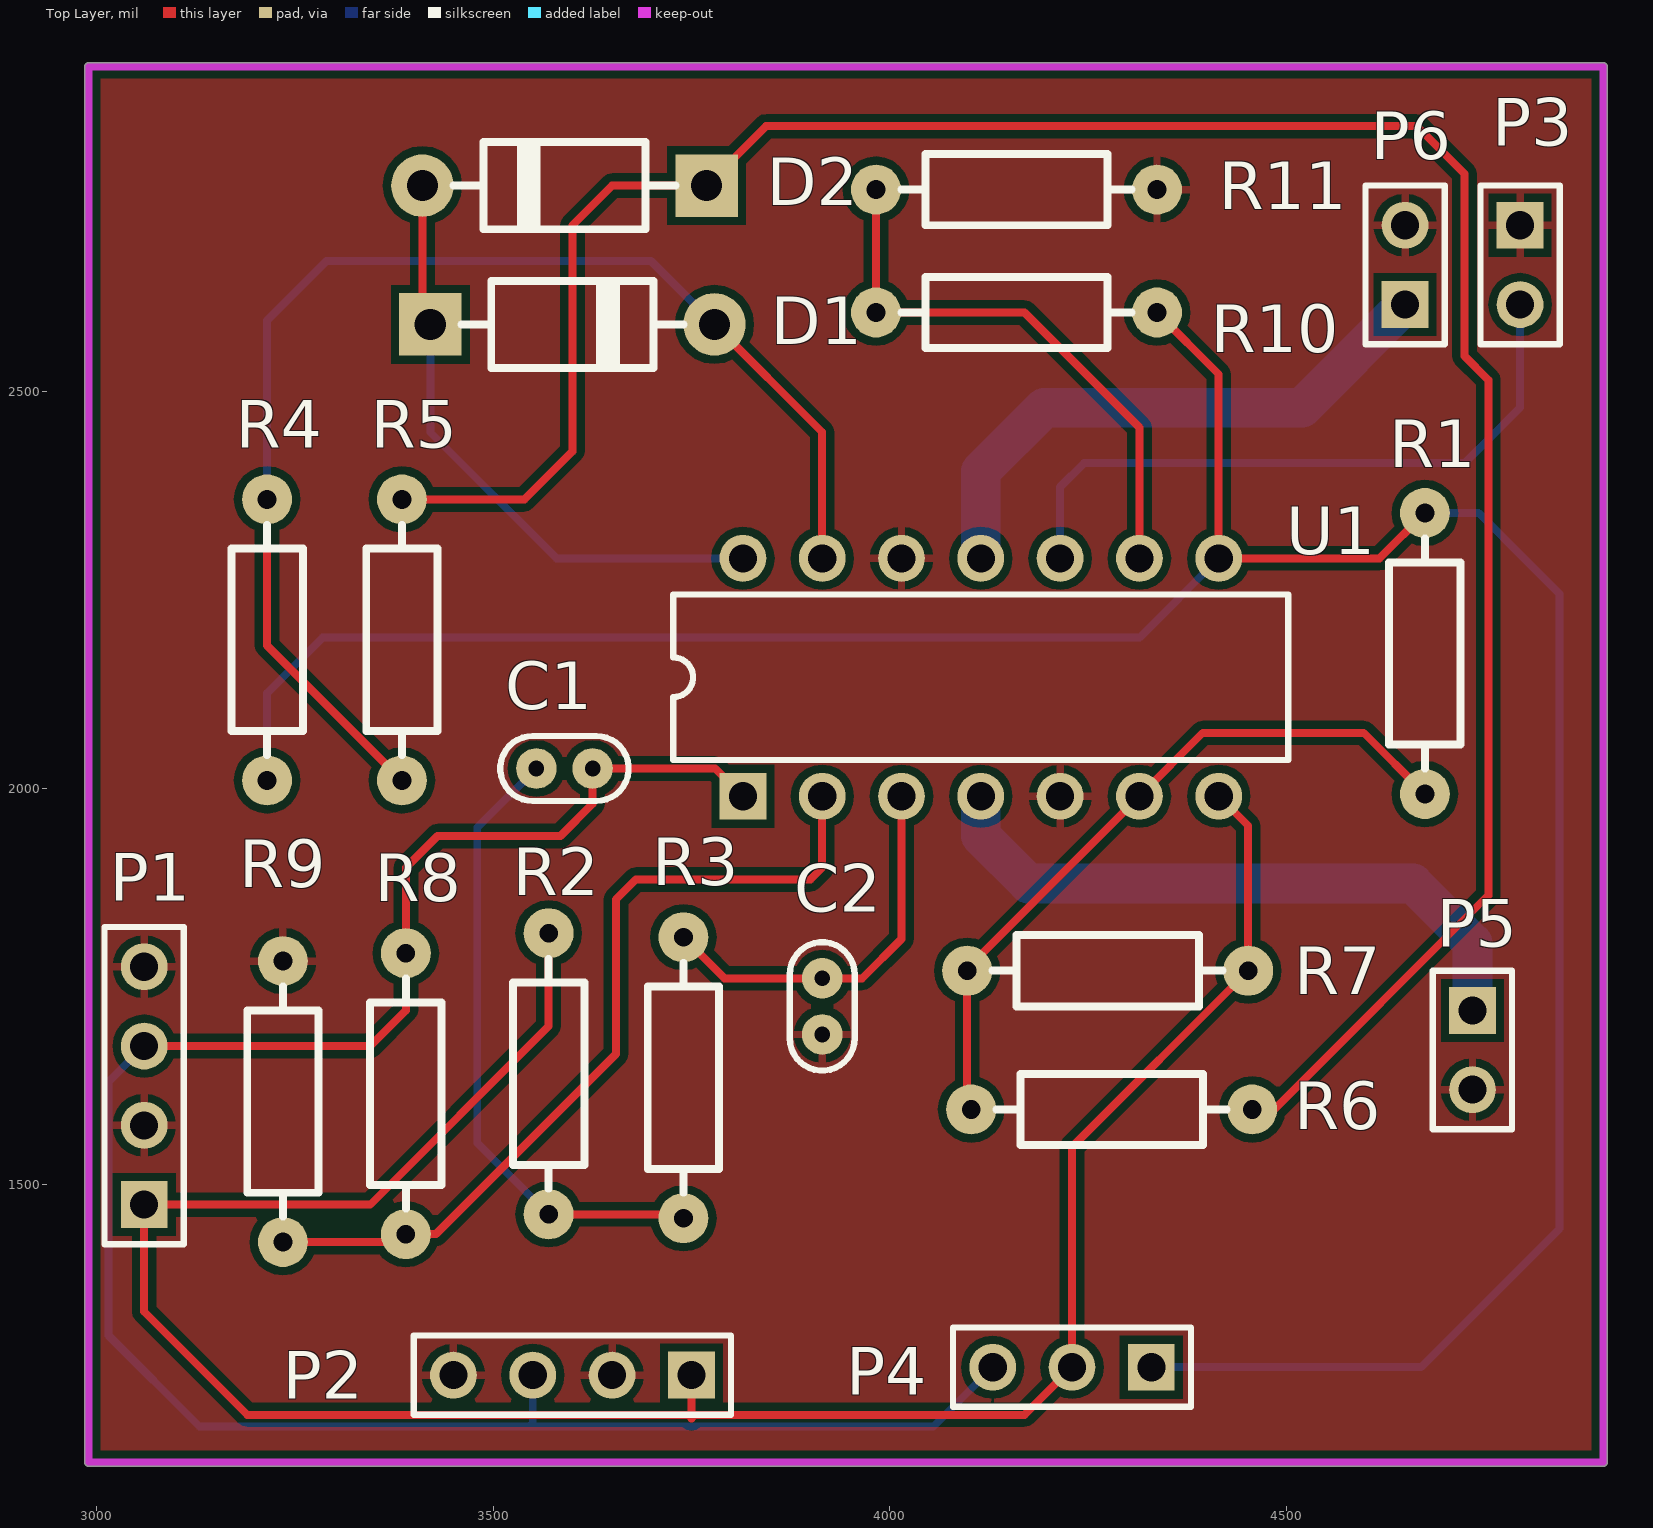
[diagram p0: Top Layer view]
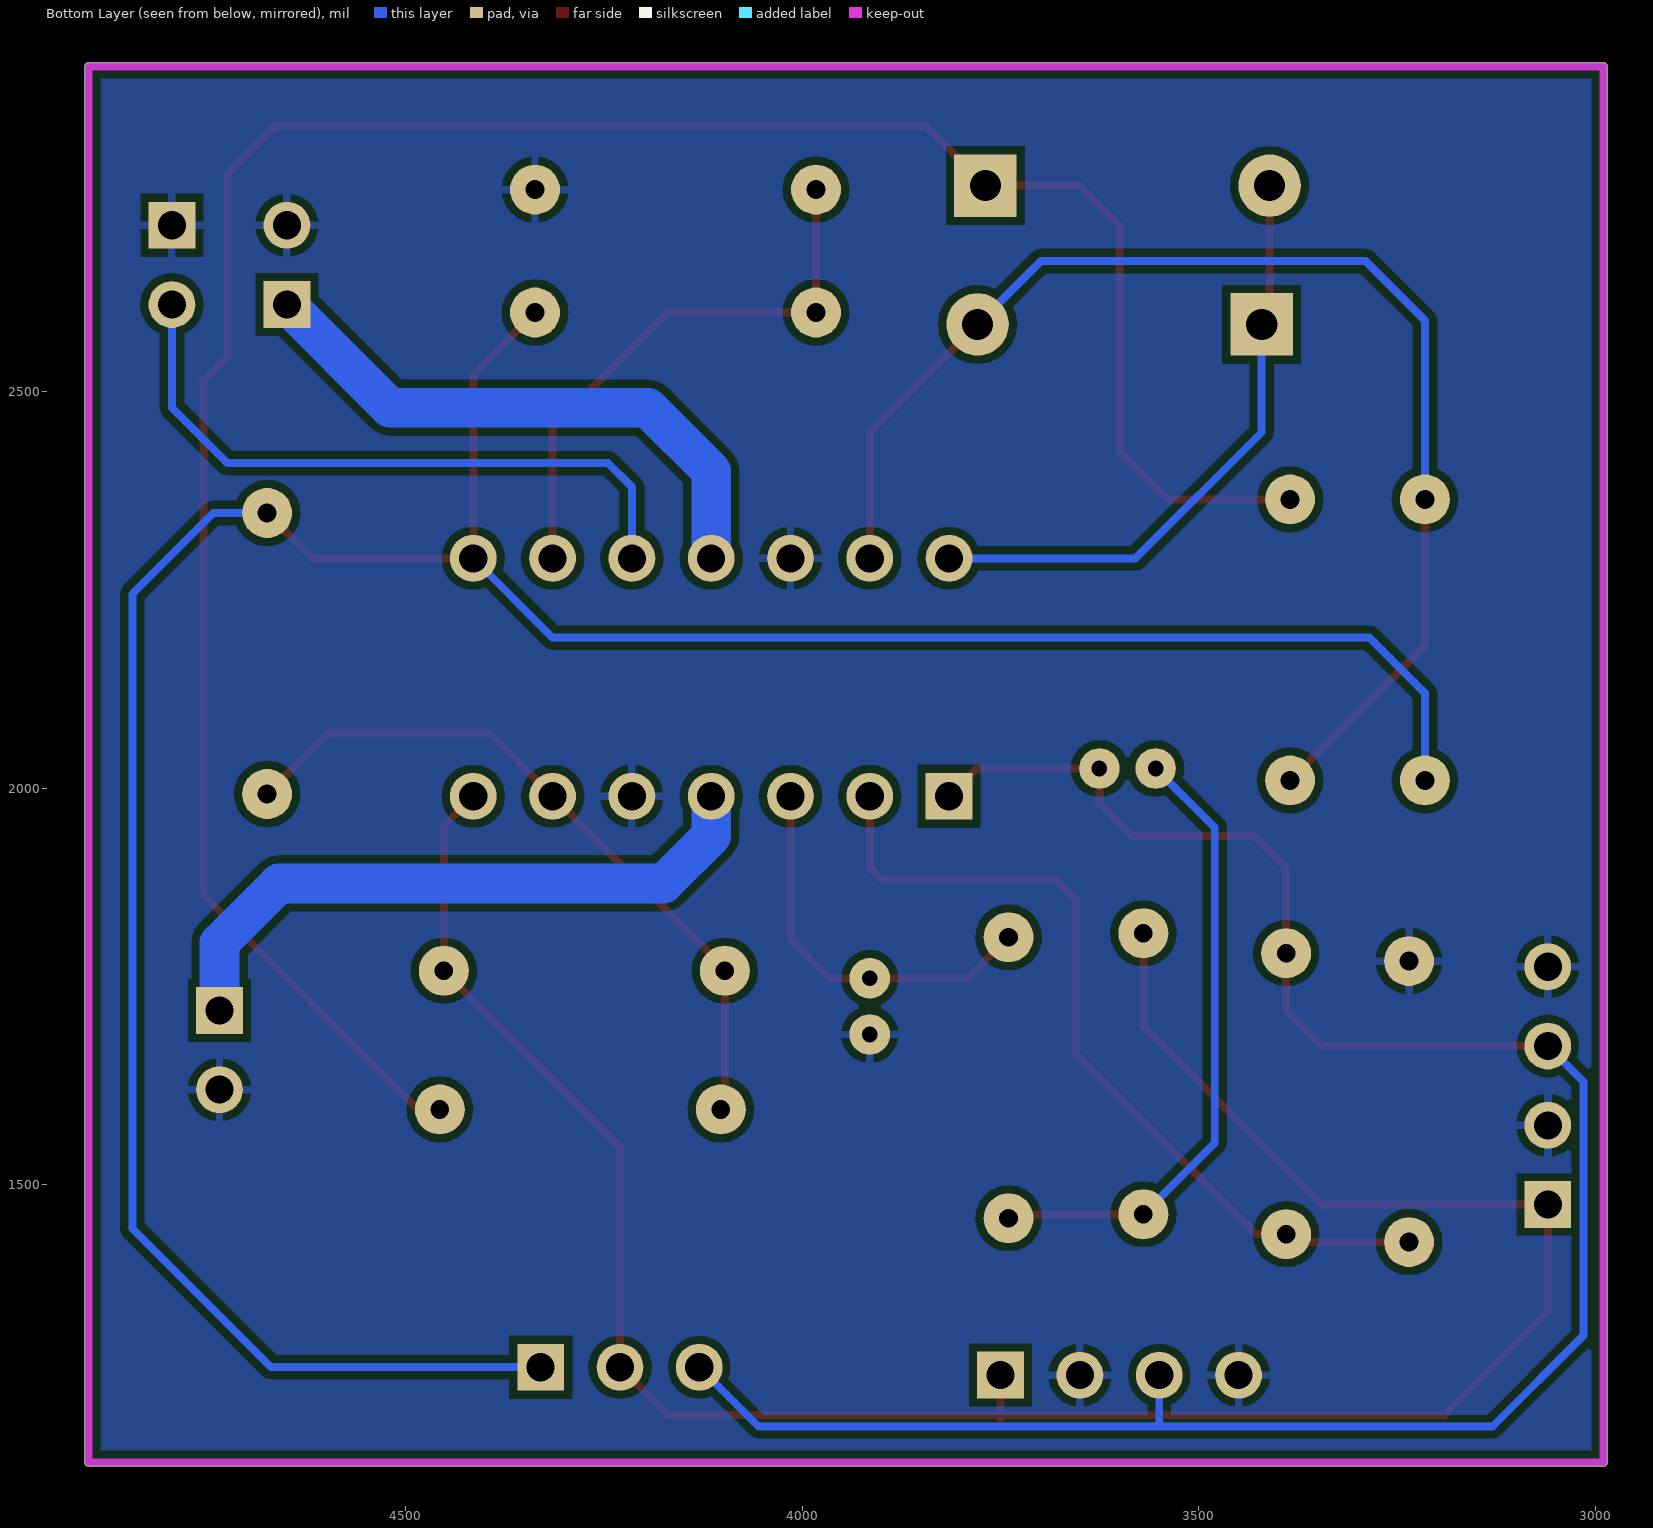
[diagram p1: Bottom Layer view, seen from below]
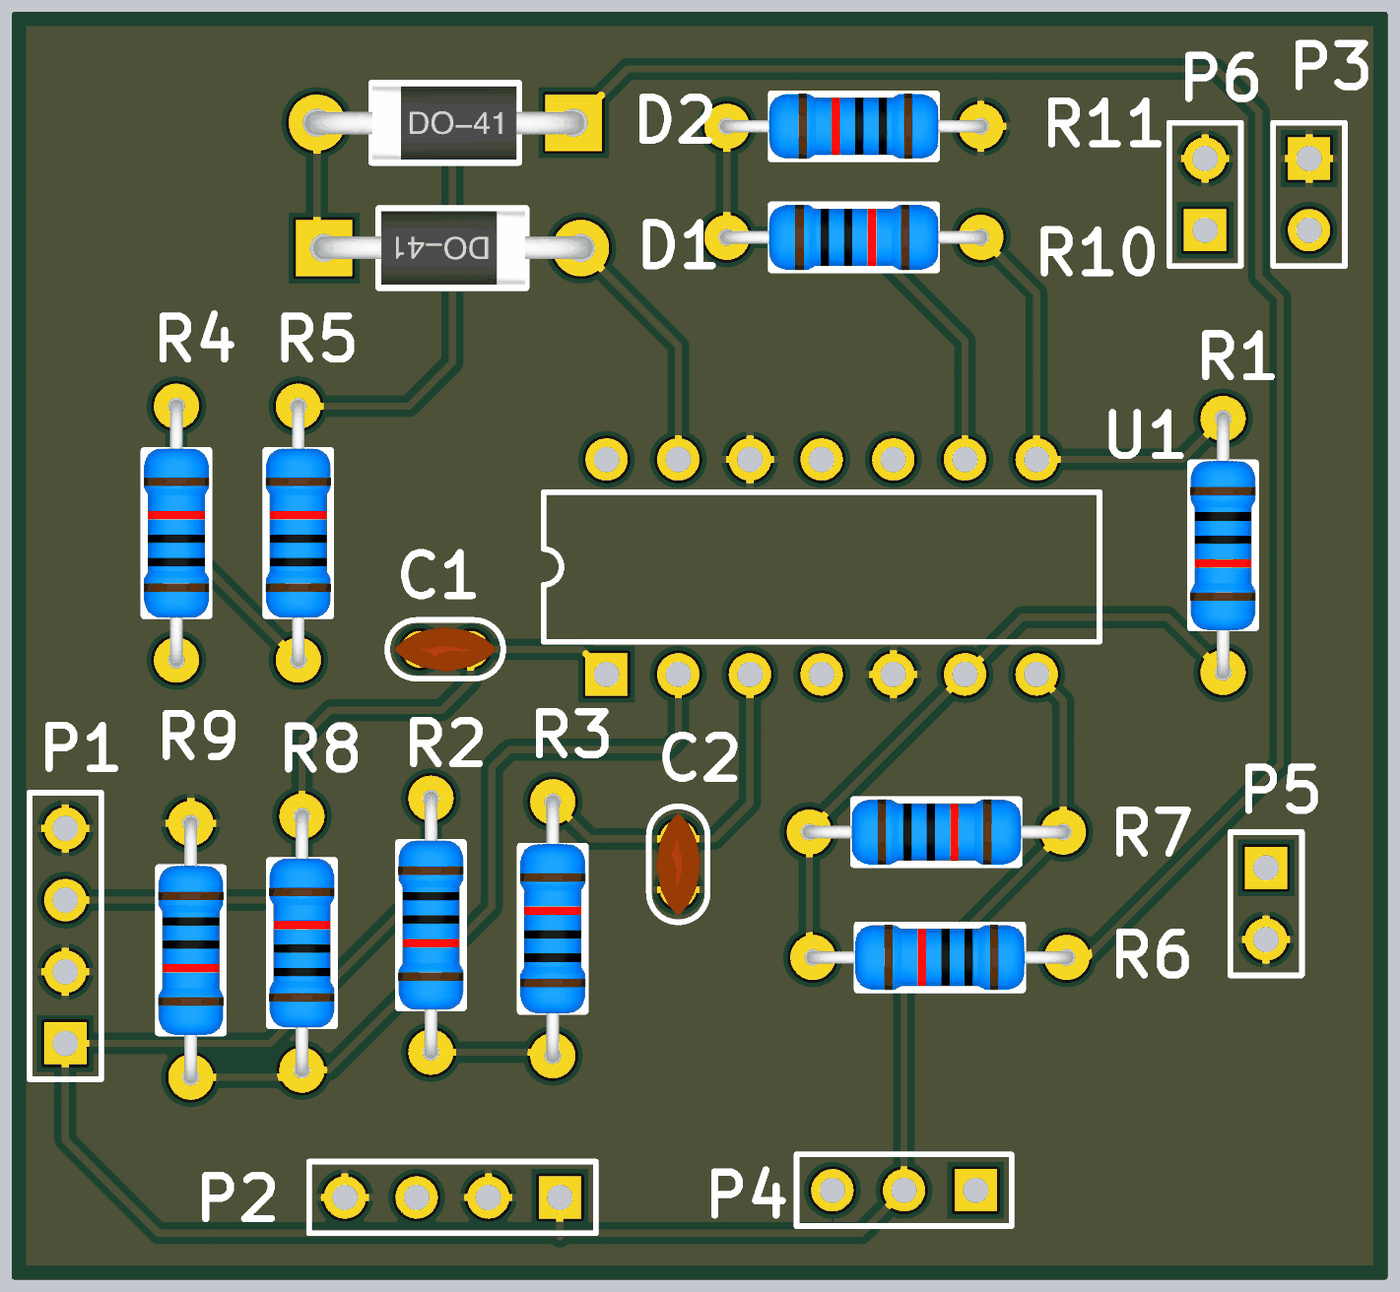
[diagram p2: 3D render of the assembled board from above, using the file's embedded part models]
# Altium PCB MISC82775.PcbDoc
Units mil, origin at the board's own origin, x right, y up, seen from the top; angles counter-clockwise.
Board outline 1920.03 x 1770.03 mil, 2 copper layers (Top Layer, Bottom Layer); 22 components, 15 nets, 61 pads, 0 vias.

## Layer stack, top to bottom (the 12.6 mil dielectric is the usual default, probably not edited)
Top Solder: solder mask 0.4, Solder Resist, Dk 3.5
Top Layer: signal copper 1.4
Dielectric 1: dielectric 12.6, FR-4, Dk 4.8
Bottom Layer: signal copper 1.4
Bottom Solder: solder mask 0.4, Solder Resist, Dk 3.5

## Board outline
2984.99,1150 ccw(c2990,1150) 2990,1144.98 4900,1144.98 ccw(c4900,1150) 4905.02,1150 4905.02,2910 ccw(c4900,2910) 4900,2915.01 2990,2915.01 ccw(c2990,2910) 2984.99,2910

## Design rules (kind name [scope] priority, off if disabled: settings)
Clearance [All] p1: gap=10
MinimumSolderMaskSliver [All] p1: minsoldermaskwidth=0
PolygonConnect [All] p1: connectstyle=Relief reliefconductorwidth=10 reliefentries=4 polygonreliefangle="90 Angle" airgapwidth=10
RoutingVias [All] p1: holewidth=28 width=50 viastyle="Through Hole" minholewidth=28 minwidth=50 maxholewidth=28 maxwidth=50
SilkToSilkClearance [All] p1: silktosilkclearance=0
SilkToSolderMaskClearance [IsPad] p1: minsilkscreentomaskgap=0 clearancetoexposedcopper=TRUE
SolderMaskExpansion [All] p1: expansion=4
Width [All] p1: maxlimit=50 minlimit=10 preferedwidth=10
27 further rules are at their usual default settings.

## Components (designator, comment, footprint, x,y, rotation, side; value= is the part's Value field where it differs from the comment)
C1 "1UF" "CC 1.8*3.6" 3590,2025 r0 top
C2 "1UF" "CC 1.8*3.6" 3915,1725 r270 top
D1 "1N4007" DO-41 3600,2585 r0 top
D2 "1N4007" DO-41 3590,2760 r180 top
P1 "Header 4" HDR1X4 3060,1475 r90 top
P2 "Header 4" HDR1X4 3750,1260 r180 top
P3 "Header 2" HDR1X2 4795,2710 r270 top
P4 "Header 3" HDR1X3 4330,1270 r180 top
P5 "Header 2" HDR1X2 4735,1720 r270 top
P6 "Header 2" HDR1X2 4650,2610 r90 top
R1 "20K" "RS 1/4W" 4675,2170 r270 top
R2 "20K" "RS 1/4W" 3570,1640 r270 top
R3 "20K" "RS 1/4W" 3740,1635 r90 top
R4 "10K" "RS 1/4W" 3215,2187.17 r90 top
R5 "10K" "RS 1/4W" 3385,2187.17 r90 top
R6 "10K" "RS 1/4W" 4280,1595 r180 top
R7 "20K" "RS 1/4W" 4275,1770 r0 top
R8 "22K" "RS 1/4W" 3390,1615 r90 top
R9 "22K" "RS 1/4W" 3235,1605 r270 top
R10 "1K" "RS 1/4W" 4160,2600 r0 top
R11 "1K" "RS 1/4W" 4160,2755 r180 top
U1 "LM224N" 646-06 4115,2140 r0 top

## Footprints (in the part's own frame and the unit in brackets; to place one, negate y for a bottom-side part, rotate by r counter-clockwise, add the part's x,y. Pads: shape width x height; smd on the part's side, far side on the other; paste and mask are expansions set on the pad)
646-06 [mm] "DIP; 14 Leads; Row Spacing 7.62 mm; Pitch 2.54 mm"
  rect 1.5x1.5 hole 0.9: 1(-7.62,-3.81)
  round 1.5 hole 0.9: 2(-5.08,-3.81) 3(-2.54,-3.81) 4(0,-3.81) 5(2.54,-3.81) 6(5.08,-3.81) 7(7.62,-3.81) 8(7.62,3.81) 9(5.08,3.81) 10(2.54,3.81) 11(0,3.81) 12(-2.54,3.81) 13(-5.08,3.81) 14(-7.62,3.81)
  silkscreen extent -9.85,-2.65 9.85,2.65
"CC 1.8*3.6" [mm] "脚距1.8mm直径3.6mm"
  round 1.3 hole 0.5: 1(-0.9,0) 2(0.9,0)
  silkscreen extent -2.05,-1.04 2.05,1.04, body extent -1.8,-0.8 1.8,0.8, height 3.6
DO-41 [mm] "2.6*9.1mm(直径，脚距）"
  rect 2x2 hole 1: 1(-4.55,0)
  round 2 hole 1: 2(4.55,0)
  silkscreen extent -3.56,-1.4 3.56,1.4, body extent -4.92,-1.29 4.98,1.31, height 2.65
HDR1X2 [mm] "Connector; Header; 2 Position"
  rect 1.5x1.5 hole 0.9: 1(0,0)
  round 1.5 hole 0.9: 2(2.54,0)
  silkscreen extent -1.27,-1.27 3.81,1.27
HDR1X3 [mm] "Connector; Header; 3 Position"
  rect 1.5x1.5 hole 0.9: 1(0,0)
  round 1.5 hole 0.9: 2(2.54,0) 3(5.08,0)
  silkscreen extent -1.27,-1.27 6.35,1.27
HDR1X4 [mm] "Connector; Header; 4 Position"
  rect 1.5x1.5 hole 0.9: 1(0,0)
  round 1.5 hole 0.9: 2(2.54,0) 3(5.08,0) 4(7.62,0)
  silkscreen extent -1.27,-1.27 8.89,1.27
"RS 1/4W" [mm] "直插色环电阻，脚距9mm，直径2.3mm"
  round 1.6 hole 0.6: 1(-4.5,0) 2(4.5,0)
  silkscreen extent -3.68,-1.14 3.68,1.14, body extent -4.72,-1.16 4.73,1.16, height 2.32

## Part data
C1 C2: library part CC, "Ceramic capacitor"
D1 D2: "Rectifier diode"
P1 P2: "Header, 4-Pin"
P3 P5 P6: "Header, 2-Pin"
P4: "Header, 3-Pin"
R1 R2 R3 R4 R5 R6 R7 R8 R9 R10 R11: library part R-S, "Color-band resistor"
U1: "Quad Low-Power Operational Amplifier"

## Nets (pads, with @x,y where several pads share a name; then routed paths per layer and width w, separated by ;. In a path a pad name is that pad's centre, name@x,y a point inside that pad or via, vN(x,y) a via of type N, cw(c..) or ccw(c..) an arc to the next point about the centre after c; other vN are vias at no path point)
+12V: P5.1 U1.4 | length 810.9
  Bottom Layer w50: U1.4 4115,1940 4175,1880 4660,1880 4735,1805 P5.1
-12V: P6.1 U1.11 | length 732
  Bottom Layer w50: U1.11 4115,2400 4195,2480 4520,2480 P6.1
GND: C2.2 P1.2 P1.4 P2.2 P2.4 P3.1 P5.2 P6.2 R9.1 R11.1 U1.5 U1.12
NetC1_1: C1.1 R2.2 R3.1 | length 802.4
  Top Layer w10: R2.2 3735,1462.83 R3.1
  Bottom Layer w10: C1.1 3480,1950.43 3480,1552.83 R2.2
NetC1_2: C1.2 P1.3 P2.3 P4.3 R8.2 U1.1 | length 2690.4
  Top Layer w10: P1.3 3345,1675 3390,1720 R8.2 3390,1900 3430,1940 3585,1940 3625.43,1980.43 C1.2 3780,2025 U1.1
  Bottom Layer w10: P1.3 3015,1630 3015,1310 3130,1195 3545,1195 ; P2.3 3550,1200 3545,1195 ; P4.3 4055,1195 3545,1195
NetC2_1: C2.1 R3.2 U1.3 | length 497
  Top Layer w10: R3.2 3791.73,1760.43 C2.1 3965.43,1760.43 4015,1810 U1.3
NetD1_1: D1.1 D2.2 U1.14 | length 775.1
  Top Layer w10: D2.2 3410.87,2595 D1.1
  Bottom Layer w10: D1.1 3420.87,2449.13 3580,2290 U1.14
NetD1_2: D1.2 R4.2 R5.1 U1.13 | length 1630
  Top Layer w10: R4.2 3215,2180 R5.1 ; D1.2 3915,2449.13 U1.13
  Bottom Layer w10: R4.2 3215,2590 3290,2665 3699.13,2665 D1.2
NetD2_1: D2.1 R5.2 R6.1 | length 3058.9
  Top Layer w10: R5.2 3539.33,2364.33 3600,2425 3600,2710 3650,2760 D2.1 3844.13,2835 4665,2835 4725,2775 4725,2545 4755,2515 4755,1865 4485,1595 R6.1
NetP1_1: P1.1 P2.1 P4.2 R2.1 R7.2 U1.7 | length 2988.6
  Top Layer w10: R2.1 3570,1700 3345,1475 P1.1 3060,1340 3190,1210 3750,1210 ; P2.1 3750,1210 ; U1.7 4452.17,1952.83 R7.2 4230,1547.83 P4.2 4170,1210 3755,1210 3750,1205 3750,1210
NetP3_2: P3.2 U1.10 | length 841.4
  Bottom Layer w10: U1.10 4215,2380 4245,2410 4725,2410 4795,2480 P3.2
NetP4_1: P4.1 R1.1 R4.1 R10.2 U1.8 | length 3606.1
  Top Layer w10: R10.2 4415,2522.17 U1.8 4617.83,2290 R1.1
  Bottom Layer w10: R4.1 3215,2120 3285,2190 4315,2190 U1.8 ; P4.1 4670,1270 4845,1445 4845,2245 4742.83,2347.17 R1.1
NetR1_2: R1.2 R6.2 R7.1 U1.6 | length 912.1
  Top Layer w10: R6.2 4097.83,1600 R7.1 4097.83,1772.83 U1.6 4395,2070 4597.83,2070 R1.2
NetR8_1: R8.1 R9.2 U1.2 | length 1079.8
  Top Layer w10: R9.2 3380,1427.83 R8.1 3427.83,1437.83 3655,1665 3655,1860 3680,1885 3900,1885 3915,1900 U1.2
NetR10_1: R10.1 R11.2 U1.9 | length 712.2
  Top Layer w10: R11.2 R10.1 4170,2600 4315,2455 U1.9

## Polygon pours and split planes (outlines as drawn)
GND on Top Layer "D" (solid, remove dead copper, pour order 0): 2725,3050 2785,3110 5350,3110 5350,1240 5025,915 4940,1000 2725,1000
GND on Bottom Layer "D" (solid, remove dead copper, pour order 2): 2535,2985 4895,2985 5085,3175 5050,3140 5050,1005 2620,1005 2615,1010

## Keep-outs
Keep-Out Layer:
  lines w10: 2990,2700 2990,2910 4900,2910 4900,1150 2990,1150 2990,2805